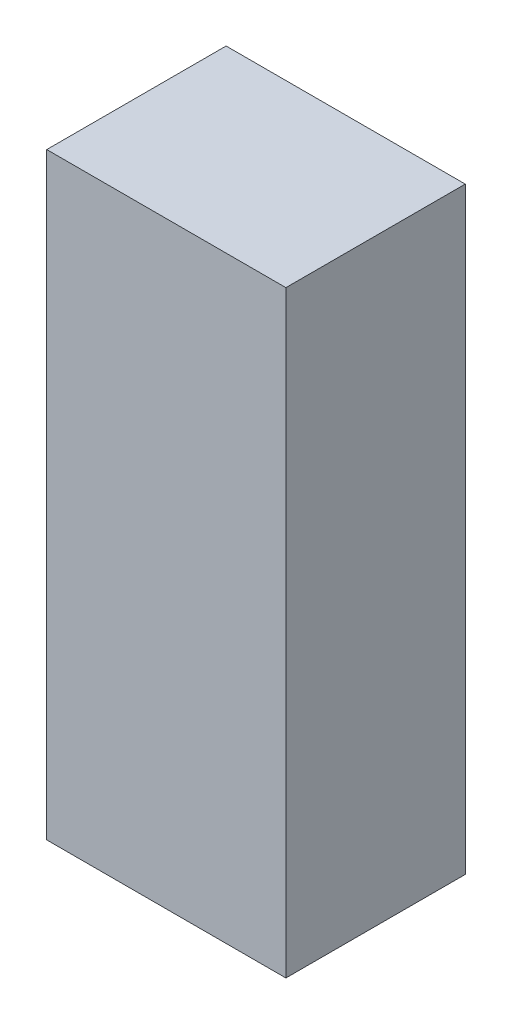
SolidWorks part; units mm, degrees
ref_plane "Front Plane" through (0, 0, 0) normal (0, 0, 1) x (1, 0, 0)
ref_plane "Top Plane" through (0, 0, 0) normal (0, 1, 0) x (1, 0, 0)
ref_plane "Right Plane" through (0, 0, 0) normal (1, 0, 0) x (0, 0, -1)
other "Configuration Table"
sketch "Sketch1" plane through (0, 0, 0) normal (0, 0, 1) x (1, 0, 0)
  line L13 (0, 0) -> (20, 0)
  line L14 (0, 0) -> (0, 50)
  line L15 (0, 50) -> (20, 50)
  line L16 (20, 0) -> (20, 50)
  dimension "D1" = 20
  dimension "D2" = 50
extrude "Boss-Extrude1" add sketch "Sketch1" along normal blind 15
